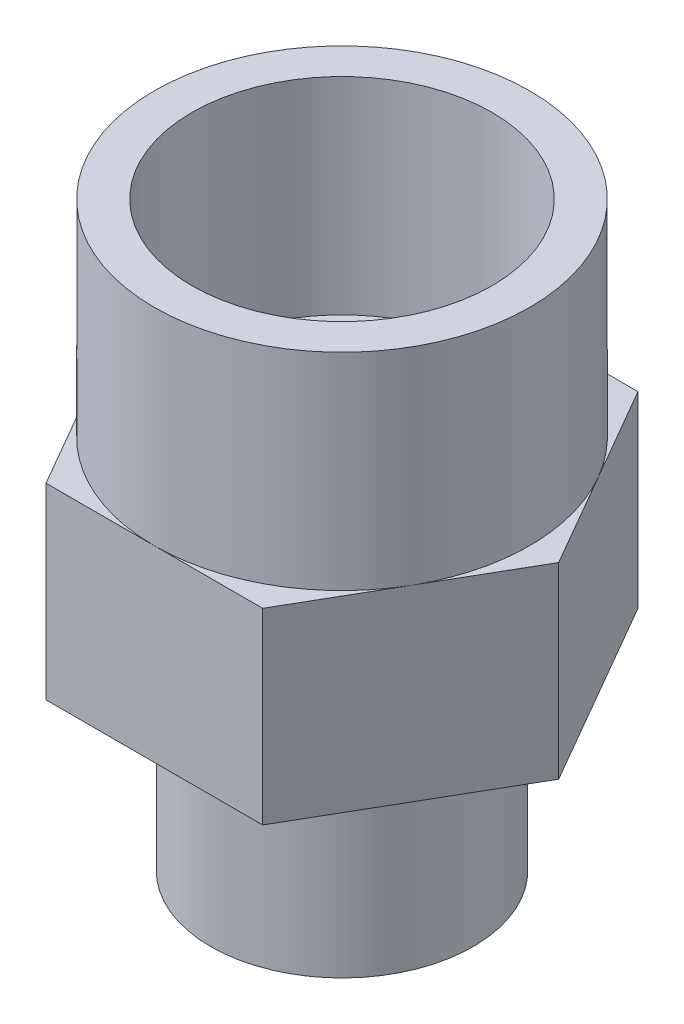
SolidWorks part; units mm, degrees
material "铜"
ref_plane "前视基准面" through (0, 0, 0) normal (0, 0, 1) x (1, 0, 0)
ref_plane "上视基准面" through (0, 0, 0) normal (0, 1, 0) x (1, 0, 0)
ref_plane "右视基准面" through (0, 0, 0) normal (1, 0, 0) x (0, 0, -1)
sketch "草图1" plane through (0, 0, 0) normal (0, 1, 0) x (1, 0, 0)
  circle A0 centre (0, 0) radius 10
  dimension "D1" = 20
extrude "拉伸-薄壁1" add sketch "草图1" along normal blind 11 thin thin type one direction reverse wall 2
sketch "草图2" plane through (0, 0, 0) normal (0, -1, 0) x (1, 0, 0)
  line L1 (11.547, 0) -> (5.7735, 10)
  line L2 (5.7735, 10) -> (-5.7735, 10)
  line L3 (-5.7735, 10) -> (-11.547, 0)
  line L4 (-11.547, 0) -> (-5.7735, -10)
  line L5 (-5.7735, -10) -> (5.7735, -10)
  line L6 (5.7735, -10) -> (11.547, 0)
  circle A0 centre (0, 0) radius 5
  circle A1 centre (0, 0) radius 10 construction
  dimension "D1" = 10
  dimension "D2" = 20
extrude "凸台-拉伸1" add sketch "草图2" along normal blind 10
sketch "草图3" plane through (0, -10, 0) normal (0, -1, 0) x (1, 0, 0)
  circle A0 centre (0, 0) radius 5
  dimension "D1" = 10
extrude "拉伸-薄壁2" add sketch "草图3" along normal blind 10 thin
